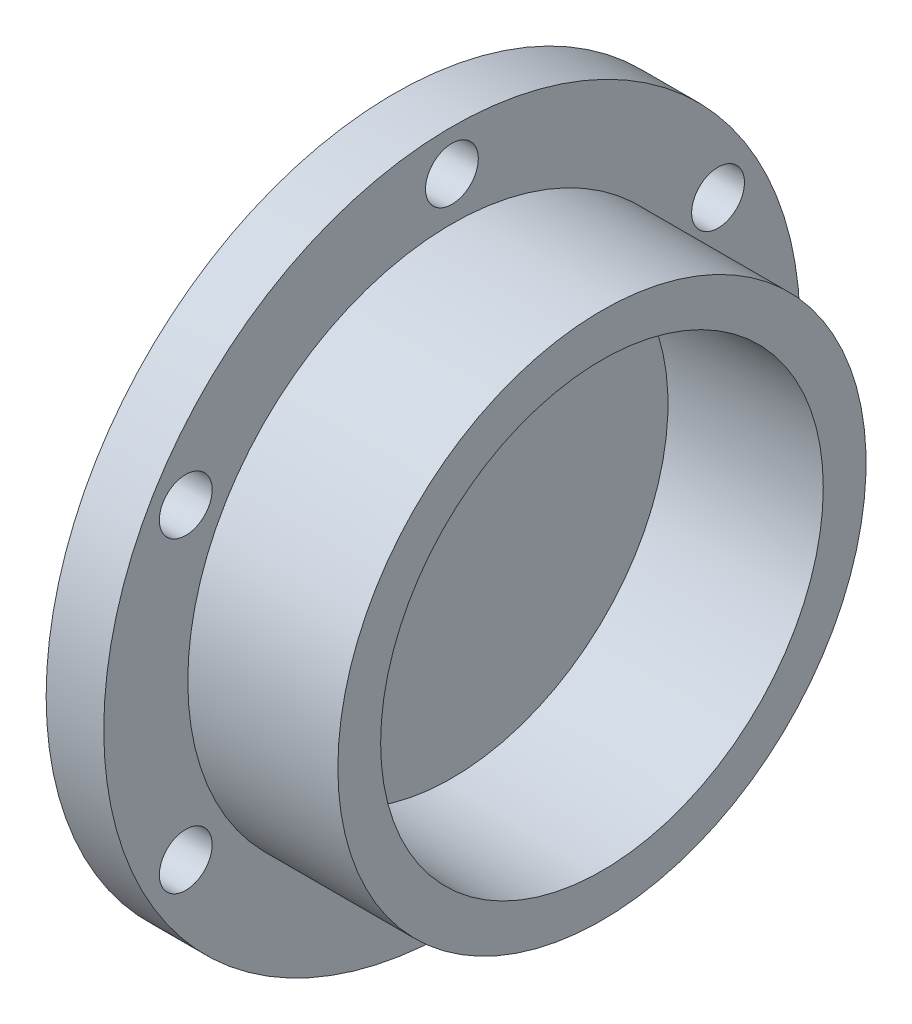
from build123d import *

# Parameters (mm, degrees)
SKETCH2_R          = 5.5
CUT_EXTRUDE1_DEPTH = 108.18704446
CIRPATTERN1_COUNT  = 6
DRAFT1_ANGLE       = 2


with BuildPart() as part:
    # Sketch1 → Revolve1 (revolve)
    with BuildSketch(Plane.XY, mode=Mode.PRIVATE) as revolve1_sk:
        Polygon((0, 0), (0, 72.5), (12, 72.5), (12, 55), (43.25, 55), (43.25, 45), (12, 45), (12, 0), align=None)
    revolve(revolve1_sk.sketch.rotate(Axis((0, 0, 0), (1, 0, 0)), 90), axis=Axis((0, 0, 0), (1, 0, 0)))

    # Sketch2 → Cut-Extrude1 (cut, through all)
    with BuildSketch(Plane(origin=(12, 0, 0), x_dir=(0, 0, -1), z_dir=(1, 0, 0))):
        with Locations((0, 64)):
            Circle(SKETCH2_R)
    cut_extrude1 = extrude(amount=-CUT_EXTRUDE1_DEPTH, mode=Mode.SUBTRACT)

    # CirPattern1: Cut-Extrude1 ×6 about axis
    cirpattern1_axis = Axis((0, 0, 0), (1, 0, 0))
    for i in range(1, CIRPATTERN1_COUNT):
        add(cut_extrude1.rotate(cirpattern1_axis, i * 360 / CIRPATTERN1_COUNT), mode=Mode.SUBTRACT)

    # Draft1
    draft1_faces = [part.faces().sort_by_distance(p)[0] for p in [
        (27.625, 0, -45),
    ]]
    draft(draft1_faces, Plane(origin=(12, 45, 0), x_dir=(0, 0, 1), z_dir=(1, 0, 0)), DRAFT1_ANGLE)


solid = part.part
